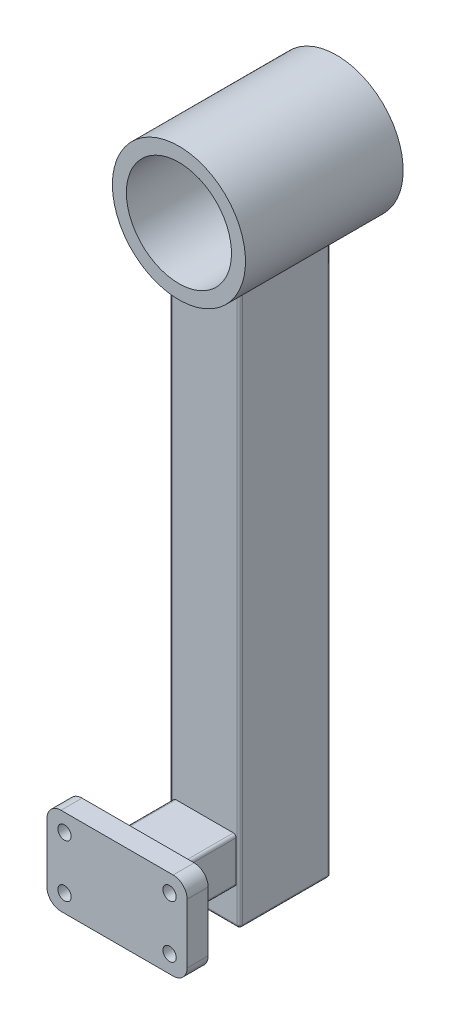
SolidWorks part; units mm, degrees
ref_plane "Front Plane" through (0, 0, 0) normal (0, 0, 1) x (1, 0, 0)
ref_plane "Top Plane" through (0, 0, 0) normal (0, 1, 0) x (1, 0, 0)
ref_plane "Right Plane" through (0, 0, 0) normal (1, 0, 0) x (0, 0, -1)
other "Configuration Table"
sketch "Sketch1" plane through (0, 0, 0) normal (0, 0, 1) x (1, 0, 0)
  line L1 (-16, 12.5) -> (16, 12.5)
  line L2 (-20, 8.5) -> (-20, -8.5)
  line L3 (-16, -12.5) -> (16, -12.5)
  line L4 (20, 8.5) -> (20, -8.5)
  line L5 (-20, 12.5) -> (20, -12.5) construction
  line L6 (-20, -12.5) -> (20, 12.5) construction
  line L9 (0, 0) -> (0, 12.5) construction
  line L10 (-15, 7.5) -> (15, 7.5) construction
  line L13 (0, 0) -> (-20, 0) construction
  line L14 (-15, 7.5) -> (-15, -7.5) construction
  line L15 (-15, -7.5) -> (15, -7.5) construction
  line L16 (15, 7.5) -> (15, -7.5) construction
  line L17 (-15, 7.5) -> (15, -7.5) construction
  line L18 (-15, -7.5) -> (15, 7.5) construction
  arc A5 (-20, -8.5) -> (-16, -12.5) centre (-16, -8.5) ccw
  arc A6 (16, -12.5) -> (20, -8.5) centre (16, -8.5) ccw
  arc A7 (16, 12.5) -> (20, 8.5) centre (16, 8.5) cw
  arc A8 (-16, 12.5) -> (-20, 8.5) centre (-16, 8.5) ccw
  circle A9 centre (-15, 7.5) radius 1.9
  circle A10 centre (15, 7.5) radius 1.9
  circle A11 centre (15, -7.5) radius 1.9
  circle A12 centre (-15, -7.5) radius 1.9
  point P0 (0, 0)
  dimension "D4" = 30
  dimension "D5" = 3.8
  dimension "D7" = 4
  dimension "D1" = 40
  dimension "D2" = 25
  dimension "D3" = 15
extrude "Boss-Extrude1" add sketch "Sketch1" along normal blind 6
sketch "Sketch2" plane through (0, 0, 0) normal (0, 0, -1) x (-1, 0, 0)
  line L0 (0, -12.5) -> (0, 12.5) construction
  line L1 (-9, 6.5) -> (9, 6.5)
  line L2 (-9, 6.5) -> (-9, -6.5)
  line L3 (-9, -6.5) -> (9, -6.5)
  line L4 (9, 6.5) -> (9, -6.5)
  line L5 (-9, 6.5) -> (9, -6.5) construction
  line L6 (-9, -6.5) -> (9, 6.5) construction
  line L7 (16, -12.5) -> (-16, -12.5) construction
  line L8 (-16, 12.5) -> (16, 12.5) construction
  point P0 (0, 0)
  dimension "D1" = 6
  dimension "D2" = 18
  dimension "D3" = 6
extrude "Boss-Extrude2" add sketch "Sketch2" along normal blind 32
sketch "Sketch4" plane through (0, -6.5, 0) normal (0, -1, 0) x (-1, 0, 0)
  line L0 (-9, 32) -> (9, 32) construction
  line L1 (10, 19) -> (-10, 19)
  line L2 (10, 19) -> (10, 45)
  line L3 (10, 45) -> (-10, 45)
  line L4 (-10, 19) -> (-10, 45)
  line L5 (10, 19) -> (-10, 45) construction
  line L6 (10, 45) -> (-10, 19) construction
  point P0 (0, 32)
  dimension "D1" = 20
  dimension "D2" = 26
extrude "Boss-Extrude3" add sketch "Sketch4" along normal blind 10 and the other way blind 150
sketch "Sketch5" plane through (0, 0, -45) normal (0, 0, -1) x (-1, 0, 0)
  line L0 (10, 143.5) -> (-10, 143.5) construction
  circle A0 centre (-1.6619, 158.5) radius 15
  circle A1 centre (-1.6619, 158.5) radius 19
  dimension "D1" = 30
  dimension "D2" = 38
  dimension "D3" = 15
extrude "Boss-Extrude4" add sketch "Sketch5" along normal blind 10 and the other way blind 35
fillet "Fillet1" radius 0.8 12 edges at (9, 6.5, -9.5) (9, -6.5, -9.5) (-9, -6.5, -9.5) (-9, 6.5, -9.5) (0, -16.5, -19) (10, 62.4637, -19) (10, 62.4637, -45) (0, -16.5, -45) (10, -16.5, -32) (-10, -16.5, -32) (-10, 63.5, -19) (-10, 63.5, -45)
